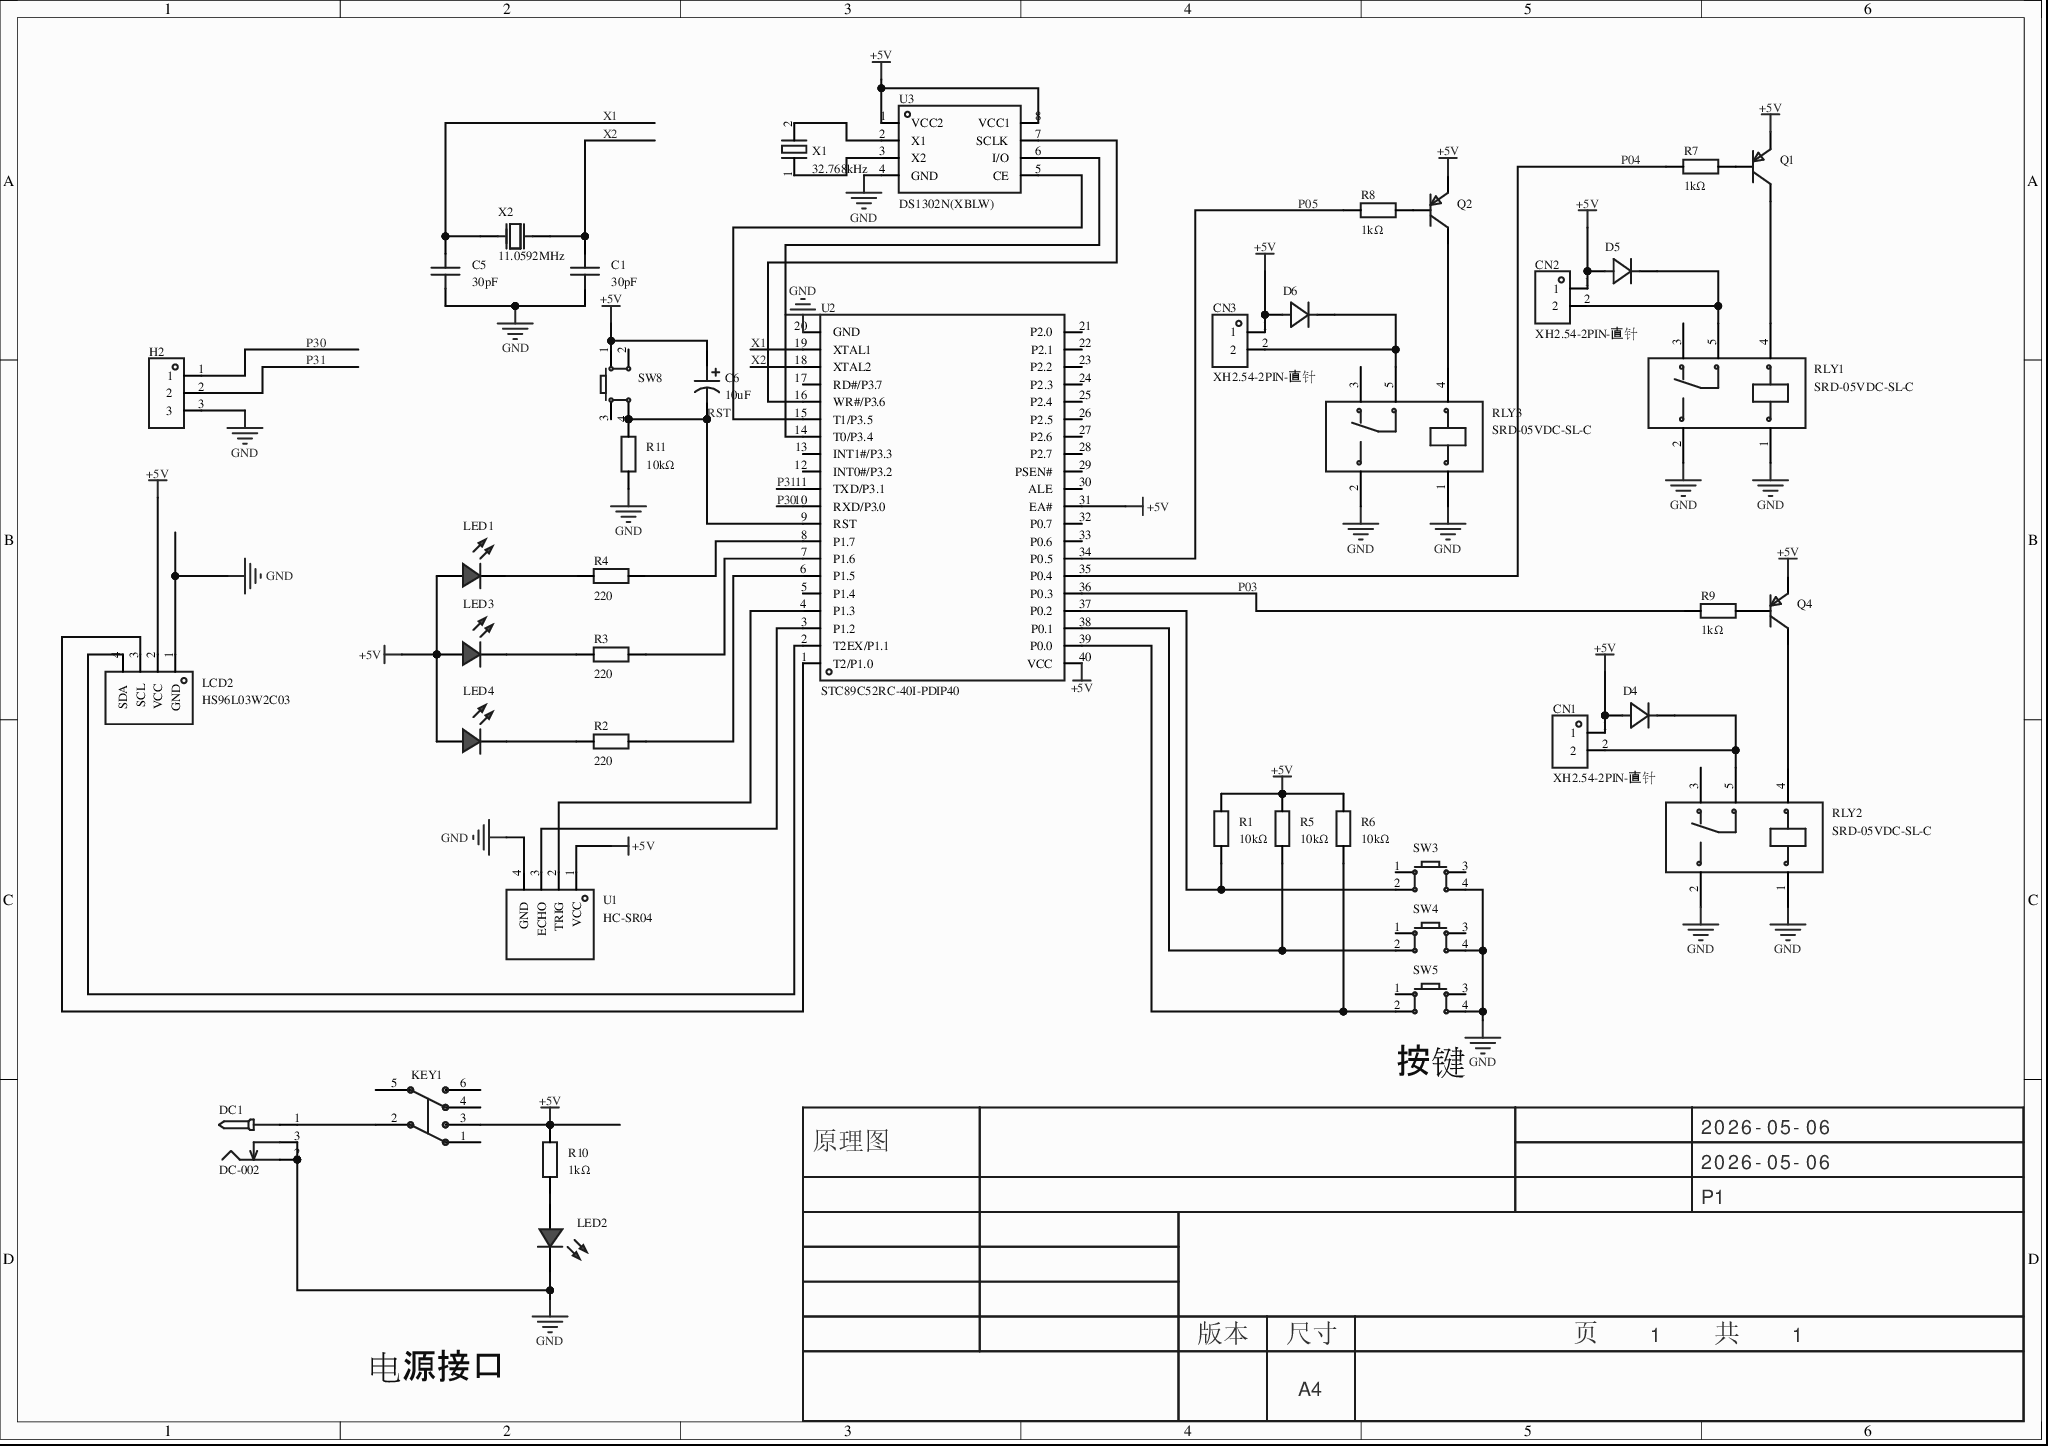
[diagram p0: MISC52010-3.schdoc]
# Altium project MISC52010-2.PrjPcb
1 sheet, 43 parts. Net scope: global (net labels, ports and power ports of the same name join across sheets).
Board file: MISC52010.pcbdoc

## Sheet MISC52010-3.schdoc
size 297 x 209 mm; Version: V1.0; @Project Name: MISC52010; @Update Date: 2026-05-06; @Create Date: 2026-05-06; @Board Name: MISC52010; @Create Time: 15:23:10; @Page Count: 1; @Page No: 1; @Schematic Name: MISC52010; @Update Time: 15:23:10; Size: A4

### Parts
C1  30pF  [CAP-TH_L3.8-W2.5-P2.54-D0.50]
C5  30pF  [CAP-TH_L3.8-W2.5-P2.54-D0.50]
C6  10uF  [CAP-TH_BD5.0-P2.00-D0.8-FD-10UF50VC110GL]
CN1  XH2.54-2PIN-直针  [CONN-TH_XH2.54-2P]
CN2  XH2.54-2PIN-直针  [CONN-TH_XH2.54-2P]
CN3  XH2.54-2PIN-直针  [CONN-TH_XH2.54-2P]
D4  (no value)  [DO_1N4007]
D5  (no value)  [DO_1N4007]
D6  (no value)  [DO_1N4007]
DC1  DC-002  [DC-IN-TH_DC-3510]
H2  (no value)  [HDR-TH_3P-P2.54-V-M]
KEY1  无自锁开关 8.5×8.5 无声  [SW-TH_6P-L8.5-W8.5-P2.54]  (value not drawn)
LCD2  HS96L03W2C03  [OLED-TH_L27.8-W27.2-P2.54_C9900033791]
LED1  (no value)  [LED_TH-3mm]
LED2  (no value)  [LED_TH-3mm]
LED3  (no value)  [LED_TH-3mm]
LED4  (no value)  [LED_TH-3mm]
Q1  (no value)  [S8550P_TO-92]
Q2  (no value)  [S8550P_TO-92]
Q4  (no value)  [S8550P_TO-92]
R1  10kΩ  [Res_1/8W]
R2  220  [R0603]
R3  220  [R0603]
R4  220  [R0603]
R5  10kΩ  [Res_1/8W]
R6  10kΩ  [Res_1/8W]
R7  1kΩ  [Res_1/8W]
R8  1kΩ  [Res_1/8W]
R9  1kΩ  [Res_1/8W]
R10  1kΩ  [Res_1/8W]
R11  10kΩ  [Res_1/8W]
RLY1  SRD-05VDC-SL-C  [RELAY-TH_SRD-XXVDC-XL-C]
RLY2  SRD-05VDC-SL-C  [RELAY-TH_SRD-XXVDC-XL-C]
RLY3  SRD-05VDC-SL-C  [RELAY-TH_SRD-XXVDC-XL-C]
SW3  (no value)  [SW-TH_4P-L6.0-W6.0-P4.50-LS6.5]
SW4  (no value)  [SW-TH_4P-L6.0-W6.0-P4.50-LS6.5]
SW5  (no value)  [SW-TH_4P-L6.0-W6.0-P4.50-LS6.5]
SW8  (no value)  [SW-TH_4P-L6.0-W6.0-P4.50-LS6.5]
U1  HC-SR04  [TH_HC-SR04V]
U2  STC89C52RC-40I-PDIP40  [DIP-40_L52.0-W13.7-P2.54-LS15.2-BL]
U3  DS1302N(XBLW)  [PDIP-8_L9.3-W6.4-P2.54-LS7.6-BL]
X1  32.768kHz  [CRYSTAL-TH_BD1.4-P0.45-D0.2]
X2  11.0592MHz  [OSC-TH_L11.1-W4.7-P4.88]

### Nets
+5V: C6.1 CN1.1 CN2.1 CN3.1 D4.2(A) D5.2(A) D6.2(A) KEY1.3 LCD2.2(VCC) LED1.1(C) LED3.1(C) LED4.1(C) Q1.1(E) Q2.1(E) Q4.1(E) R1.2 R5.2 R6.2 R10.2 SW8.1 U1.1(VCC) U2.31(EA#) U2.40(VCC) U3.1(VCC2) U3.8(VCC1)
GND: C1.1 C5.1 DC1.2 DC1.3 H2.3 LCD2.1(GND) LED2.2(A) R11.1 RLY1.1 RLY1.2 RLY2.1 RLY2.2 RLY3.1 RLY3.2 SW3.4 SW4.4 SW5.4 U1.4(GND) U2.20(GND) U3.4(GND)
P03: R9.2 U2.36(P0.3)
P04: R7.2 U2.35(P0.4)
P05: R8.2 U2.34(P0.5)
P30: H2.1 U2.10(RXD/P3.0)
P31: H2.2 U2.11(TXD/P3.1)
RST: C6.2 R11.2 SW8.4 U2.9(RST)
X1: C5.2 U2.19(XTAL1) X2.1(OSC1)
X2: C1.2 U2.18(XTAL2) X2.2(OSC2)
NetCN1_2: CN1.2 D4.1(K) RLY2.5
NetCN2_2: CN2.2 D5.1(K) RLY1.5
NetCN3_2: CN3.2 D6.1(K) RLY3.5
NetDC1_1: DC1.1 KEY1.2
NetLCD2_3: LCD2.3(SCL) U2.1(T2/P1.0)
NetLCD2_4: LCD2.4(SDA) U2.2(T2EX/P1.1)
NetLED1_2: LED1.2(A) R4.1
NetLED2_1: LED2.1(C) R10.1
NetLED3_2: LED3.2(A) R3.1
NetLED4_2: LED4.2(A) R2.1
NetQ1_2: Q1.2(B) R7.1
NetQ1_3: Q1.3(C) RLY1.4
NetQ2_2: Q2.2(B) R8.1
NetQ2_3: Q2.3(C) RLY3.4
NetQ4_2: Q4.2(B) R9.1
NetQ4_3: Q4.3(C) RLY2.4
NetR1_1: R1.1 SW3.2 U2.37(P0.2)
NetR2_2: R2.2 U2.6(P1.5)
NetR3_2: R3.2 U2.7(P1.6)
NetR4_2: R4.2 U2.8(P1.7)
NetR5_1: R5.1 SW4.2 U2.38(P0.1)
NetR6_1: R6.1 SW5.2 U2.39(P0.0)
NetU1_2: U1.2(TRIG) U2.4(P1.3)
NetU1_3: U1.3(ECHO) U2.3(P1.2)
NetU2_14: U2.14(T0/P3.4) U3.6(I/O)
NetU2_15: U2.15(T1/P3.5) U3.5(CE)
NetU2_16: U2.16(WR#/P3.6) U3.7(SCLK)
NetU3_2: U3.2(X1) X1.2
NetU3_3: U3.3(X2) X1.1

Not connected (* = marked no-connect by the designer): KEY1 1 4 5 6; RLY1 3; RLY2 3; RLY3 3; SW3 1 3; SW4 1 3; SW5 1 3; SW8 2 3; U2 5(P1.4) 12(INT0#/P3.2) 13(INT1#/P3.3) 17(RD#/P3.7) 21(P2.0) 22(P2.1) 23(P2.2) 24(P2.3) 25(P2.4) 26(P2.5) 27(P2.6) 28(P2.7) 29(PSEN#) 30(ALE) 32(P0.7) 33(P0.6)

### Notes on the sheet
- (near SW5) 按键
- 电源接口
- 2026-05-06
- 原理图
- P1
- 版本
- 尺寸
- A4
- 页    1    共    1

### Library data of the parts
C1 C5 = C315C300K3G5TA7301: 容值:30pF;精度:±10%;额定电压:25V;温度系数:C0G;; Manufacturer: KEMET(基美); 3D Model: 0be8c650c9044d099e9add656cc6dda60819f05c4eef4c71ace90d822a990e87; 3D Model Transform: 149.606,98.8187,0,0,0,0,0,0,-196.85; Tolerance: ±10%; Voltage Rating: 25V; Temperature Coefficient: C0G; Pin Spacing: 2.54mm; AddInBom: yes; Symbol: C315C300K3G5TA7301; Device: C315C300K3G5TA7301; LCSC Part Name: 30pF ±10% 25V; Supplier Part: C2245291; Manufacturer Part: C315C300K3G5TA7301; Supplier Footprint: 插件,P=2.54mm; JLCPCB Part Class: Extended Part; Datasheet: https://item.szlcsc.com/datasheet/C315C300K3G5TA7301/2337370.html; Supplier: LCSC; Value: 30pF; ConvertToPcb: yes; FootprintName: CAP-TH_L3.8-W2.5-P2.54-D0.50; ModelName: CAP-TH_L3.8-W2.5-P2.54-D0.50
C6 = 10UF50VC110GL: 容值:10uF;精度:±20%;额定电压:50V;纹波电流:120mA@100KHz;等效串联电阻(ESR):1.6Ω;; Manufacturer: Econd(米朗电子); Tolerance: ±20%; Voltage Rating: 50V; Equivalent Series Resistance(ESR): 1.6Ω; Pin Spacing: 2mm; Lifetime: 5000hrs@105℃; AddInBom: yes; Symbol: 10UF50VC110GL; Device: 10UF50VC110GL; LCSC Part Name: 10uF ±20% 50V; Supplier Part: C46867109; Manufacturer Part: 10UF50VC110GL; Supplier Footprint: 插件,D5xL11mm; JLCPCB Part Class: Extended Part; Datasheet: https://item.szlcsc.com/datasheet/10UF50VC110GL/49031974.html; Supplier: LCSC; Value: 10uF; Ripple Current: 120mA@100KHz; Diameter: 5mm; Height - Seated (Max): 11mm; Operating Temperature: -40℃~+105℃; ConvertToPcb: yes; FootprintName: CAP-TH_BD5.0-P2.00-D0.8-FD-10UF50VC110GL
CN1-CN3 = XH2.54-2PIN-直针: AddInBom: yes; ModelId: c3cc11bd8b8748c1ae6bc231aac3a1ff0819f05c4eef4c71ace90d822a990e87; ModelTransform: 296.889,230.315,0,0,0,0,0,26.653,-137.795; Symbol: XH2.54-2PIN-直针; Device: XH2.54-2PIN-直针; LCSC Part Name: XH2.54-2PIN-直针; SupplierPart: C9900011425; ManufacturerPart: XH2.54-2PIN-直针; Supplier Footprint: XH2.54-2PIN; JLCPCB Part Class: Extended Part; Supplier: LCSC; ConvertToPcb: yes; FootprintName: CONN-TH_XH2.54-2P; ModelName: CONN-TH_XH2.54-2P
D4-D6 = D_1N4007A: AddInBom: yes; ModelId: 6de1e9b71a0d4751b4e9df530304c1a30819f05c4eef4c71ace90d822a990e87; ModelName: DO-41_D2.4-L4.7-P8.70; ModelTransform: 373.9,94.4,232.29,0,0,0,0,0,-140; Symbol: D_1N4007; Device: D_1N4007A; Supplier Footprint: DO-41; ConvertToPcb: yes; FootprintName: DO_1N4007
DC1 = DC-002: 3D Model: 28059cb5f325411c86e5e1af88d5b1310819f05c4eef4c71ace90d822a990e87; 3D Model Transform: 450.787,208.661,0,180,0,0,113.189,-47.244,-125.984; AddInBom: yes; Symbol: DC-002; Device: DC-002; LCSC Part Name: DC-002 铁脚 内铁芯1.0mm; Supplier Part: C12568; Manufacturer Part: DC-002; Supplier Footprint: 插件; JLCPCB Part Class: Extended Part; Supplier: LCSC; ConvertToPcb: yes; FootprintName: DC-IN-TH_DC-3510; ModelName: DC-IN-TH_DC-3510
H2 = HDR-M_2.54_1x3P: 3D Model: bb473b6d38ff42a99216a4fcdbdcc4cb0819f05c4eef4c71ace90d822a990e87; 3D Model Transform: 300.03877,100,0,0,0,0,0,0,-118.11; AddInBom: yes; ModelName: HDR-TH_3P-P2.54-M-LI-1X3P; Symbol: HDR-M_2.54_1x3P; Device: HDR-M_2.54_1x3P; Supplier Part: C2937625; Supplier Footprint: 插件; ConvertToPcb: yes; FootprintName: HDR-TH_3P-P2.54-V-M
KEY1 = 无自锁开关 8.5×8.5 无声: 6脚，8.5×8.5; Symbol: No self-locking switch 8.5×8.5 silent; 3D Model: 4c72b3966b92446eb355e1bd0fb4f8800819f05c4eef4c71ace90d822a990e87; 3D Model Transform: 342.519,334.645,0,180,0,0,0,0,-137.795; AddInBom: yes; Device: 无自锁开关 8.5×8.5 无声; LCSC Part Name: 无自锁开关 8.5×8.5  无声; Supplier Part: C26228; Manufacturer Part: 无自锁开关 8.5×8.5 无声; Supplier Footprint: 插件; JLCPCB Part Class: Extended Part; Supplier: LCSC; ConvertToPcb: yes; FootprintName: SW-TH_6P-L8.5-W8.5-P2.54; ModelName: SW-TH_6P-L8.5-W8.5-P2.54
LCD2 = HS96L03W2C03: 核心芯片:SSD1315芯片;接口类型:I2C;尺寸(inch):0.96;像素分辨率:128x64;; Manufacturer: HS(汉昇); AddInBom: yes; ModelId: bb65183306db4ca69fb52250be49b00e0819f05c4eef4c71ace90d822a990e87; ModelTransform: 1070.864,1094.486,0,0,0,0,0,-498.424,0; Interface: I2C; Dot Pixels: 128x64; Type of Drive: 无源(PMOLED); Display Range: 21.744x10.864mm; Display Color: 白色; Luminance: 180cd/m2; Symbol: HS96L03W2C03; Device: HS96L03W2C03; LCSC Part Name: 0.96寸OLED显示屏窄白光IIC; SupplierPart: C5248080; ManufacturerPart: HS96L03W2C03; Supplier Footprint: -; JLCPCB Part Class: Extended Part; Datasheet: https://item.szlcsc.com/datasheet/HS96L03W2C03/5960631.html; Supplier: LCSC; ConvertToPcb: yes; FootprintName: OLED-TH_L27.8-W27.2-P2.54_C9900033791; ModelName: OLED-TH_L27.8-W27.2-P2.54_C9900033791; Controller Type: SSD1315芯片; Size: 0.96; Operating Temperature: -40℃~+70℃; Function: -; Quiescent Current: -
LED1-LED4 = LED_TH-R_3mm: 3D Model: a497c992633541038a38947cdc58012f0819f05c4eef4c71ace90d822a990e87; 3D Model Transform: 141.274,153.327,0,0,0,0,-5.984,0,-137.795; ConvertToPcb: yes; ModelName: LED-TH-3mm_R; Symbol: LED_TH-R; Device: LED_TH-R_3mm; Supplier Footprint: 插件; AddInBom: yes; FootprintName: LED_TH-3mm
Q1 Q2 Q4 = S8550_TO_PNP: 3D Model: aafe8e06f2154e7c93506efd0d6632dd0819f05c4eef4c71ace90d822a990e87; 3D Model Transform: 180.78,141.44,417.3,0,0,0,0,0,-200; ConvertToPcb: yes; ModelName: TO-92-3_L4.9-W3.7-P1.27-L; Symbol: S8550_TO_PNP; Device: S8550_TO_PNP; Supplier Footprint: TO-92; AddInBom: yes; FootprintName: S8550P_TO-92
R1 R5-R11 = Res_AXIAL-1/8W: Symbol: 电阻; 3D Model: b2b5ae7ae4c642178fe0039925c86a3f0819f05c4eef4c71ace90d822a990e87; 3D Model Transform: 282.86,66.88,253.09,0,0,0,0,0,-191; ConvertToPcb: yes; ModelName: RES-TH_BD1.8-L3.2-P7.20-D0.4; Device: Res_AXIAL-1/8W; Supplier Footprint: 轴向引线; AddInBom: yes; FootprintName: Res_1/8W
  R1 R5 R6 R11: Value: 10kΩ
  R7-R10: Value: 1kΩ
R2-R4 = Res_0603: Symbol: 电阻; ConvertToPcb: yes; ModelId: fc143cca1e79419f9cd78b61e9279f080819f05c4eef4c71ace90d822a990e87; ModelTransform: 31.8897,63.7794,0,90,0,0,0,0,0; Device: Res_0603; Value: 220; AddInBom: yes; Supplier Footprint: 0603; FootprintName: R0603; ModelName: R0603
RLY1-RLY3 = SRD-05VDC-SL-C: 线圈电压:5V;触点形式:一组转换:1C(单刀双掷-转换);触点容量(电阻负载):-;最大切换电压:250V@AC;最大切换电流:15A;; Manufacturer: 松乐; 3D Model: d0eda9b8bf8746d18ae810ab88dc78e70819f05c4eef4c71ace90d822a990e87; 3D Model Transform: 755.904,622.4397,0,0,0,0,34.882,0,-118.11; Coil Voltage: 5V; Coil Rated Power: 360mW; Switching Current(Max): 15A; Coil Type: 无极性-单线圈; Coil Resistance: 70Ω; Contact Resistance: 100mΩ; Operate Time: 10ms; AddInBom: yes; ModelName: RELAY-TH_L19.2-W15.6-H15.8; Symbol: SRD-05VDC-SL-C; Device: SRD-05VDC-SL-C; LCSC Part Name: 蓝色 单组转换型继电器; Supplier Part: C35449; Manufacturer Part: SRD-05VDC-SL-C; Supplier Footprint: 插件,19.2x15.6mm; JLCPCB Part Class: Extended Part; Datasheet: https://item.szlcsc.com/datasheet/SRD-05VDC-SL-C/36422.html; Supplier: LCSC; Contact Form: 一组转换:1C(单刀双掷-转换); Number of Pins: 5; Contact Rating: -; Switching Voltage(Max): 250V@AC; Release Time: 10ms; ConvertToPcb: yes; FootprintName: RELAY-TH_SRD-XXVDC-XL-C
SW3-SW5 SW8 = Key_TH_6x6x6: 触点电流:50mA;额定电压(DC):12V;绝缘电阻:100MΩ;电路结构:单刀单掷;安装方式:直插;按钮形状:圆形按钮;按钮/盖帽颜色:黑色;作用力:260gf@±30gf;工作温度:-25℃~+70℃;引脚样式:PC引脚;开关长度:6mm;开关宽度:6mm;开关高度:6mm;带支架:否;; Symbol: 轻触按键; 3D Model: 20eee248bc684ccd8cbdbb1d0d91ec6f0819f05c4eef4c71ace90d822a990e87; 3D Model Transform: 236.22,323.03,0,90,0,0,0,0,-137.795; AddInBom: yes; ModelName: SW-TH_4P-L6.0-W6.0-H5.0-LS6.5-P4.50; Device: Key_TH_6x6x6; Supplier Footprint: 插件; ConvertToPcb: yes; FootprintName: SW-TH_4P-L6.0-W6.0-P4.50-LS6.5
U1 = HC-SR04: Manufacturer: Universal Microelectronics; AddInBom: yes; ModelId: d459d248281f4140aaafbda3f8c1b0d5; Symbol: HC-SR04; Device: HC-SR04; LCSC Part Name: HC-SR04; SupplierPart: C19857336; ManufacturerPart: HC-SR04; Supplier Footprint: -; JLCPCB Part Class: Extended Part; Datasheet: https://item.szlcsc.com/datasheet/HC-SR04/21184790.html; Supplier: LCSC; ConvertToPcb: yes; FootprintName: TH_HC-SR04V; ModelName: HC-SR04
U2 = STC89C52RC-40I-PDIP40: CPU内核:51家族;CPU最大主频:-;; Manufacturer: STC; AddInBom: yes; ModelId: 16d4686a009b4ddca948f91eddb57b140819f05c4eef4c71ace90d822a990e87; ModelName: DIP-40_L52.3-W13.8-H4.0-LS15.24-P2.54; ModelTransform: 2059.051,615.743,0,0,0,0,0,0,-118.11; CPU Core: 51家族; Program Storage Size: 8KB; Program Memory Type: FLASH; Voltage - Supply: 3.3V~5.5V; Symbol: STC89C52RC-40I; Device: STC89C52RC-40I-PDIP40; LCSC Part Name: 单片机原理及应用; SupplierPart: C14022; ManufacturerPart: STC89C52RC-40I-PDIP40; Supplier Footprint: DIP-40; JLCPCB Part Class: Extended Part; Datasheet: https://item.szlcsc.com/datasheet/STC89C52RC-40I-PDIP40/14679.html; Supplier: LCSC; ConvertToPcb: yes; FootprintName: DIP-40_L52.0-W13.7-P2.54-LS15.2-BL; CPU Maximum Speed: -; RAM Size: -; EEPROM: -; Number of I/O: -; ADC (Bit): -; DAC (Bit): -
U3 = DS1302N(XBLW): 接口类型:三线串行接口;晶振:外置;闹钟输出:-;; Manufacturer: XBLW(芯伯乐); AddInBom: yes; ModelId: fe5fd42f66544692923c5fbf1ee41ec70819f05c4eef4c71ace90d822a990e87; ModelName: PDIP-8_L10.2-W5.9-H4.5-P2.54-LS7.6-BL; ModelTransform: 364.173,311.8104,0,0,0,0,0,0,-118.11; Interface: 三线串行接口; Voltage - Supply: 2V~5.5V; Current - Supply: 1uA; crystal oscillator: 外置; Symbol: DS1302N(XBLW); Device: DS1302N(XBLW); LCSC Part Name: DS1302N(XBLW); SupplierPart: C42395632; ManufacturerPart: DS1302N(XBLW); Supplier Footprint: DIP-8; JLCPCB Part Class: Extended Part; Datasheet: https://atta.szlcsc.com/upload/public/pdf/source/20241125/ED583BD048AAE751CB9F5E4637775452.pdf; Supplier: LCSC; ConvertToPcb: yes; FootprintName: PDIP-8_L9.3-W6.4-P2.54-LS7.6-BL; Alarm Output: -; Operating Temperature: -40℃~+85℃
X1 = AB15T-32.768KHZ: 频率:32.768kHz;常温频差:±20ppm;外接负载电容:12.5pF;频率稳定度(全温):-;; Manufacturer: ABRACON; AddInBom: yes; ModelId: 9fdeeb9d7ef84072bac6c58c302789500819f05c4eef4c71ace90d822a990e87; ModelTransform: 55.00706,55.09,0,0,0,0,0,0,-169.291; Normal temperature Frequency Tolerance: ±20ppm; External load capacitor: 12.5pF; Equivalent Series Resistance (ESR): 40kΩ; Symbol: AB15T-32.768KHZ; Device: AB15T-32.768KHZ; LCSC Part Name: 32.768kHz ±20ppm 12.5pF; SupplierPart: C1669866; ManufacturerPart: AB15T-32.768KHZ; Supplier Footprint: DT-15; JLCPCB Part Class: Extended Part; Datasheet: https://atta.szlcsc.com/upload/public/pdf/source/20210504/0EA8EED362197519A7C3815AD65C577B.pdf; Supplier: LCSC; ConvertToPcb: yes; FootprintName: CRYSTAL-TH_BD1.4-P0.45-D0.2; ModelName: CRYSTAL-TH_BD1.4-P0.45-D0.2; Value: 32.768kHz; Frequency Stability(Full temperature range): -; Operating Temperature: -20℃~+70℃
X2 = 9AC11059302060C3: 晶振类型:直插晶振;频率:11.0592MHz;常温频差:±20ppm;负载电容:30pF;; Manufacturer: JGHC(晶光华); 3D Model: f2ed30de83344a4b83b1c4b1b9fe18560819f05c4eef4c71ace90d822a990e87; 3D Model Transform: 436.37503,185.039,0,0,0,0,0,0,-137.795; Normal temperature Frequency Tolerance: ±20ppm; Load Capacitance: 30pF; Equivalent Series Resistance(ESR): 60Ω; AddInBom: yes; Symbol: 9AC11059302060C3; Device: 9AC11059302060C3; LCSC Part Name: 11.0592MHz ±20ppm 30pF; Supplier Part: C2715911; Manufacturer Part: 9AC11059302060C3; Supplier Footprint: HC-49S; JLCPCB Part Class: Extended Part; Datasheet: https://item.szlcsc.com/datasheet/9AC11059302060C3/2832137.html; Supplier: LCSC; Type: 直插晶振; Value: 11.0592MHz; Operating Temperature: -40℃~+85℃; ConvertToPcb: yes; FootprintName: OSC-TH_L11.1-W4.7-P4.88; ModelName: OSC-TH_L11.1-W4.7-P4.88